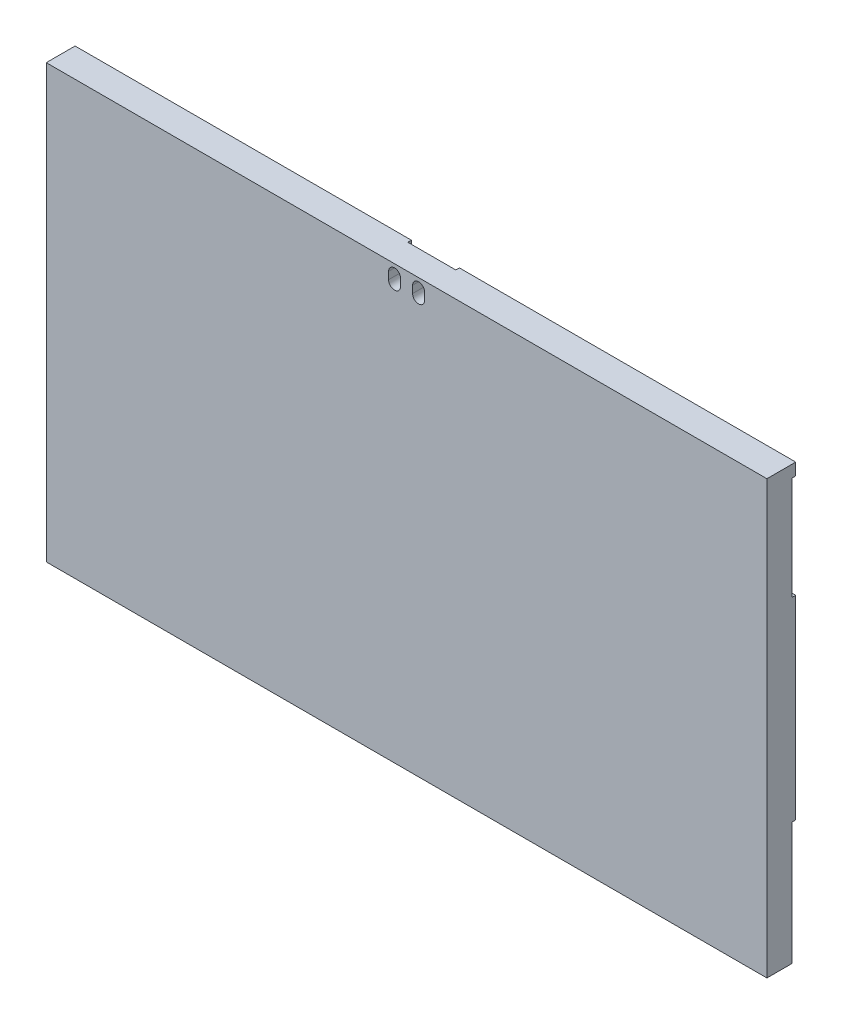
SolidWorks part; units mm, degrees
ref_plane "前视基准面" through (0, 0, 0) normal (0, 0, 1) x (1, 0, 0)
ref_plane "上视基准面" through (0, 0, 0) normal (0, 1, 0) x (1, 0, 0)
ref_plane "右视基准面" through (0, 0, 0) normal (1, 0, 0) x (0, 0, -1)
sketch "草图1" plane through (0, 0, 0) normal (0, 0, 1) x (1, 0, 0)
  line L1 (-150, -90) -> (150, -90)
  line L2 (-150, -90) -> (-150, 90)
  line L3 (-150, 90) -> (150, 90)
  line L4 (150, -90) -> (150, 90)
  line L5 (-150, -90) -> (150, 90) construction
  line L6 (-150, 90) -> (150, -90) construction
  point P0 (0, 0)
  dimension "D1" = 180
  dimension "D2" = 300
extrude "凸台-拉伸1" add sketch "草图1" along normal blind 12
sketch "草图2" plane through (0, 0, 0) normal (0, 0, -1) x (-1, 0, 0)
  line L0 (150, 90) -> (150, -90) construction
  line L1 (-150, 42) -> (150, 42)
  line L2 (-150, 42) -> (-150, 85)
  line L3 (-150, 85) -> (150, 85)
  line L4 (150, 42) -> (150, 85)
  line L5 (-150, 90) -> (150, 90) construction
  line L6 (-150, -90) -> (-150, 90) construction
  line L7 (-150, -90) -> (150, -90)
  line L8 (-150, -90) -> (-150, -39)
  line L9 (-150, -39) -> (150, -39)
  line L10 (150, -90) -> (150, -39)
  line L11 (150, -90) -> (-150, -90) construction
  dimension "D1" = 5
  dimension "D2" = 43
  dimension "D3" = 124
extrude "切除-拉伸1" cut sketch "草图2" against normal blind 1.5
sketch "草图3" plane through (0, 0, 0) normal (0, 0, -1) x (-1, 0, 0)
  line L0 (150, 85) -> (-150, 85) construction
  line L1 (-10, 85) -> (10, 85)
  line L2 (-10, 85) -> (-10, 90)
  line L3 (-10, 90) -> (10, 90)
  line L4 (10, 85) -> (10, 90)
  line L5 (-10, 85) -> (10, 90) construction
  line L6 (-10, 90) -> (10, 85) construction
  line L7 (-150, 90) -> (150, 90) construction
  point P0 (0, 87.5)
  dimension "D1" = 20
extrude "切除-拉伸2" cut sketch "草图3" against normal up to surface (1.5 mm away) up to face at (0, 63.5, 1.5)
sketch "草图4" plane through (0, 0, 1.5) normal (0, 0, -1) x (-1, 0, 0)
  line L0 (-5, 83) -> (-5, 86) construction
  line L1 (-7.5, 83) -> (-7.5, 86)
  line L2 (-2.5, 83) -> (-2.5, 86)
  line L3 (10, 90) -> (-10, 90) construction
  arc A0 (-7.5, 83) -> (-2.5, 83) centre (-5, 83) ccw
  arc A1 (-2.5, 86) -> (-7.5, 86) centre (-5, 86) ccw
  point P2 (-5, 84.5)
  dimension "D1" = 2.5
  dimension "D2" = 3
  dimension "D3" = 5
  dimension "D4" = 4
extrude "切除-拉伸3" cut sketch "草图4" against normal up to next
mirror "镜向1" about plane through (0, 0, 0) normal (1, 0, 0) of "切除-拉伸3"
